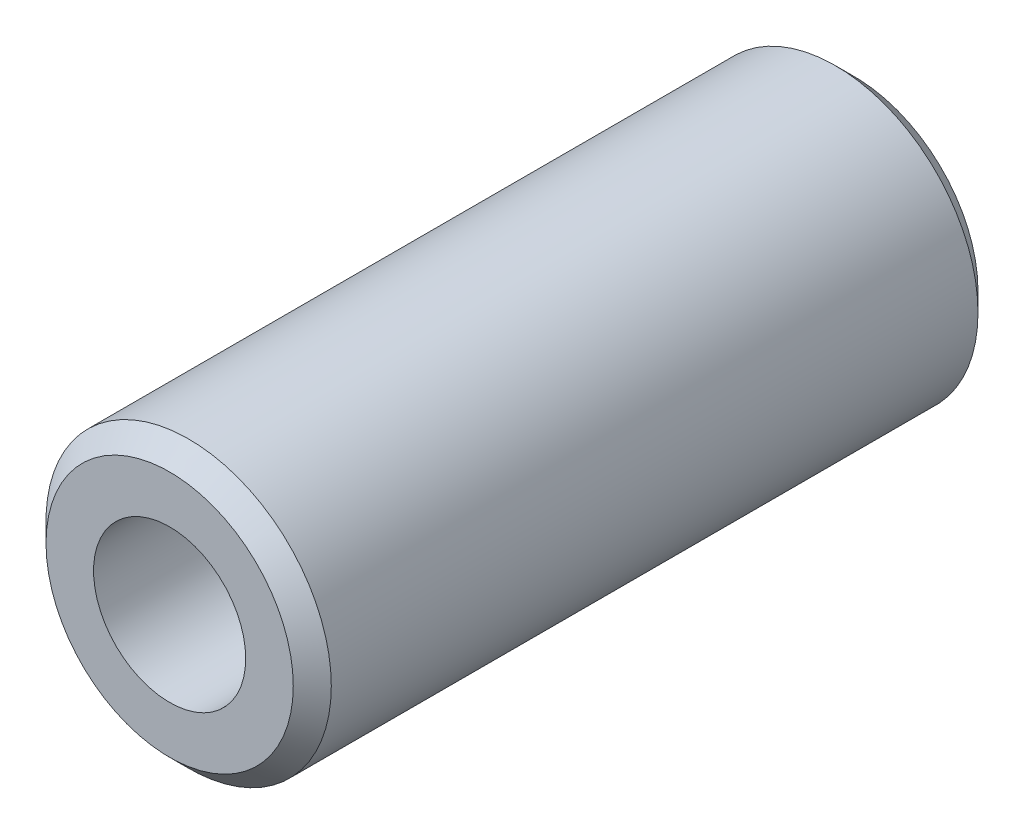
from build123d import *

# Parameters (mm, degrees)
SKETCH1_R           = 7.5
BOSS_EXTRUDE1_DEPTH = 36
CHAMFER1_SIZE       = 1
SKETCH2_R           = 4
CUT_EXTRUDE1_DEPTH  = 38.52998801


with BuildPart() as part:
    # Sketch1 → Boss-Extrude1 (new body)
    with BuildSketch(Plane.XY):
        Circle(SKETCH1_R)
    extrude(amount=BOSS_EXTRUDE1_DEPTH)

    # Chamfer1
    chamfer1_edges = [part.edges().sort_by_distance(p)[0] for p in [
        (-7.5, 0, 0),
        (-7.5, 0, 36),
    ]]
    chamfer(chamfer1_edges, length=CHAMFER1_SIZE)

    # Sketch2 → Cut-Extrude1 (cut, through all)
    with BuildSketch(Plane.XY.offset(36)):
        Circle(SKETCH2_R)
    extrude(amount=-CUT_EXTRUDE1_DEPTH, mode=Mode.SUBTRACT)


solid = part.part
